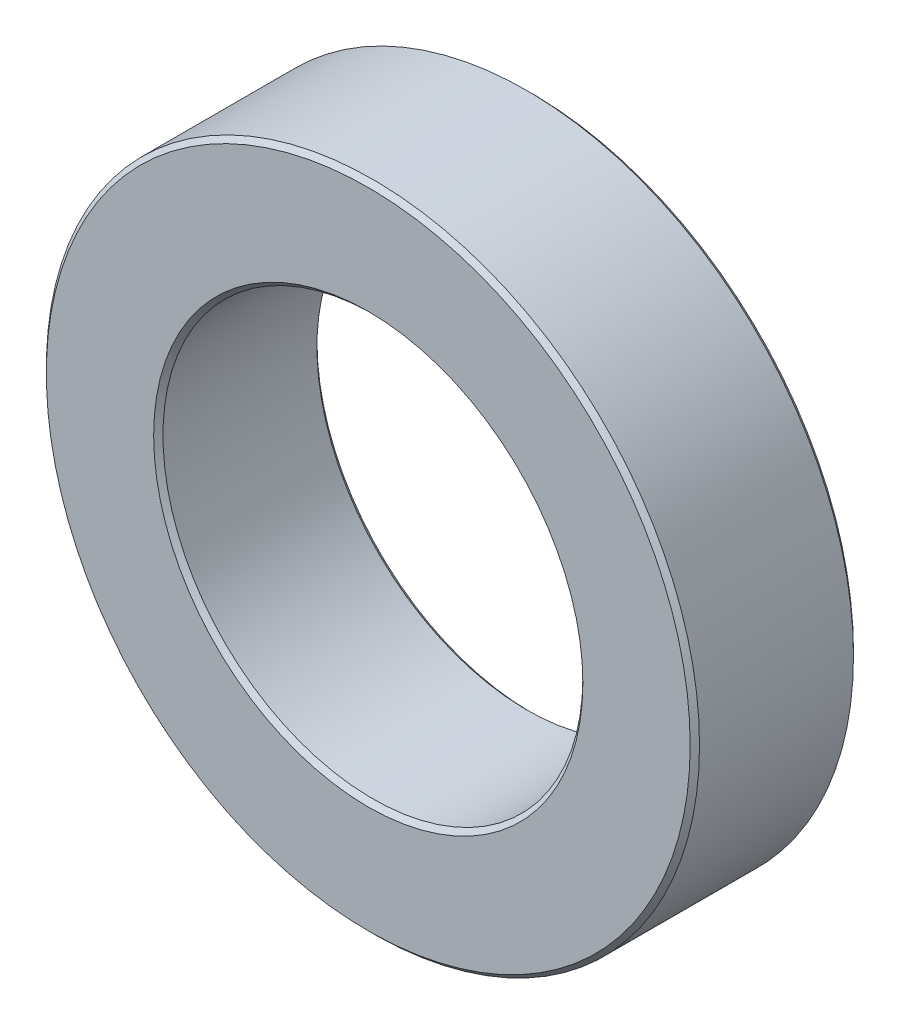
SolidWorks part; units mm, degrees
material "普通碳钢"
ref_plane "前视基准面" through (0, 0, 0) normal (0, 0, 1) x (1, 0, 0)
ref_plane "上视基准面" through (0, 0, 0) normal (0, 1, 0) x (1, 0, 0)
ref_plane "右视基准面" through (0, 0, 0) normal (1, 0, 0) x (0, 0, -1)
sketch "草图1" plane through (0, 0, 0) normal (0, 0, 1) x (1, 0, 0)
  circle A0 centre (0, 0) radius 22.5
  circle A1 centre (0, 0) radius 35
  dimension "D1" = 45
  dimension "D2" = 70
extrude "凸台-拉伸1" add sketch "草图1" along normal blind 17.5
chamfer "倒角1" distance 0.5 angle 45 4 edges at (22.5, 0, 0) (35, 0, 0) (22.5, 0, 17.5) (35, 0, 17.5)
